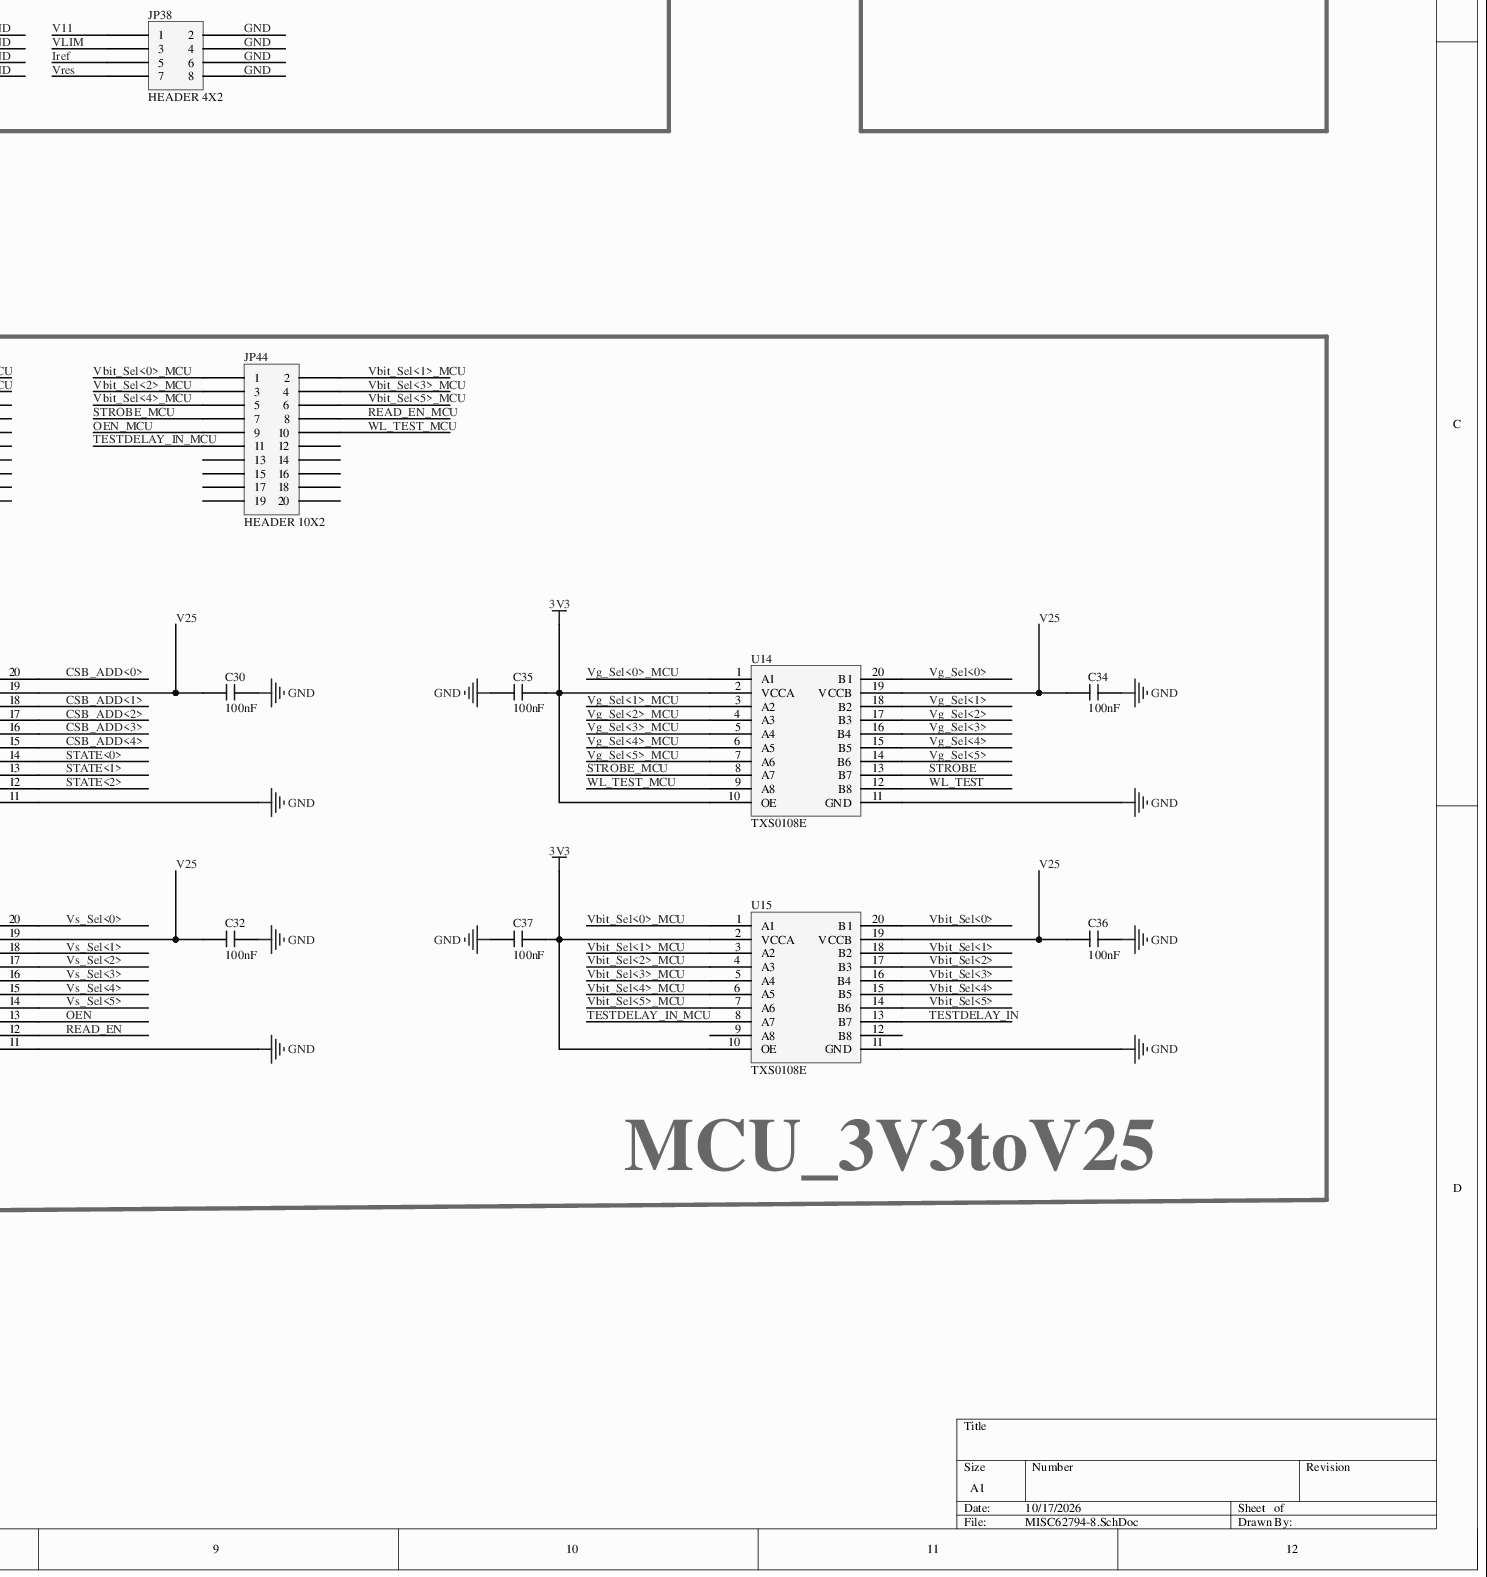
[diagram p0: MISC62794-8.SchDoc, bottom right]
# Altium project MISC62794-12.PrjPcb (part 3 of 3)

## Nets that join several sheets
GND: MISC62794-2 (36 pins), MISC62794-8 (188 pins)
USB_5V: MISC62794-2 (24 pins), MISC62794-8 (JP13.1 JP13.3)
VCC_5V: MISC62794-2 (B31.1 IC1.10 IC1.16 JP31.1), MISC62794-8 (22 pins)
DAC1: MISC62794-2 (R1.2 TP1.1 U8.1), MISC62794-8 (JP3.1)
DAC2: MISC62794-2 (R3.1 TP2.1 U8.7), MISC62794-8 (JP3.2)
DAC3: MISC62794-2 (R5.2 TP3.1 U10.1), MISC62794-8 (JP4.1)
DAC4: MISC62794-2 (R7.1 TP4.1 U10.7), MISC62794-8 (JP4.2)
DAC5: MISC62794-2 (R9.2 TP5.1 U9.1), MISC62794-8 (JP5.1)
DAC6: MISC62794-2 (R11.1 TP6.1 U9.7), MISC62794-8 (JP5.2)
DAC7: MISC62794-2 (TP7.1 U4.5), MISC62794-8 (JP7.2)
DAC8: MISC62794-2 (TP8.1 U4.8), MISC62794-8 (JP7.4)
DAC9: MISC62794-2 (TP9.1 U5.5), MISC62794-8 (JP7.6)
DAC10: MISC62794-2 (TP10.1 U5.8), MISC62794-8 (JP7.8)
DAC11: MISC62794-2 (TP11.1 U6.5), MISC62794-8 (JP7.10)
DAC12: MISC62794-2 (TP12.1 U6.8), MISC62794-8 (JP7.12)
DAC13: MISC62794-2 (R13.2 TP13.1 U11.1), MISC62794-8 (JP7.14)
DAC14: MISC62794-2 (5 pins), MISC62794-8 (JP8.1 JP8.2)